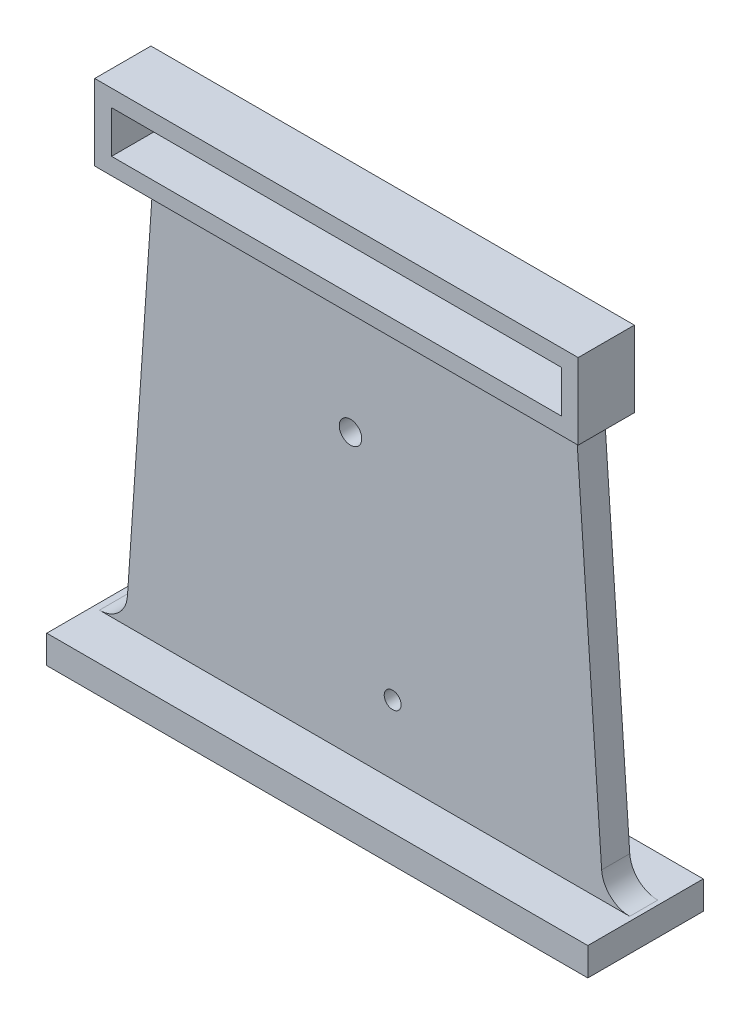
from build123d import *

# Parameters (mm, degrees)
SKETCH1_R           = 3
SKETCH1_R_2         = 4
BOSS_EXTRUDE1_DEPTH = 10
SKETCH2_W           = 192.506357526
SKETCH2_H           = 41.072090777
BOSS_EXTRUDE2_DEPTH = 10
FILLET1_R           = 10
SKETCH3_W           = 172
SKETCH3_H           = 27
SKETCH3_W_2         = 160
SKETCH3_H_2         = 15
BOSS_EXTRUDE3_DEPTH = 10


with BuildPart() as part:
    # Sketch1 → Boss-Extrude1 (new body)
    with BuildSketch(Plane.XY):
        Polygon((0, 0), (170, 0), (160, 146), (10, 146), align=None)
        with Locations((95, 24.5)):
            Circle(SKETCH1_R, mode=Mode.SUBTRACT)
        with Locations((80, 99.5)):
            Circle(SKETCH1_R_2, mode=Mode.SUBTRACT)
    extrude(amount=BOSS_EXTRUDE1_DEPTH)

    # Sketch2 → Boss-Extrude2 (add)
    with BuildSketch(Plane(origin=(0, 0, 0), x_dir=(-1, 0, 0), z_dir=(0, -1, 0))):
        with Locations((-84.638287431, -5.918559418)):
            Rectangle(SKETCH2_W, SKETCH2_H)
    extrude(amount=BOSS_EXTRUDE2_DEPTH)

    # Fillet1
    fillet1_edges = [part.edges().sort_by_distance(p)[0] for p in [
        (170, 0, 5),
        (0, 0, 5),
    ]]
    fillet(fillet1_edges, radius=FILLET1_R)

    # Sketch3 → Boss-Extrude3 (add, symmetric)
    with BuildSketch(Plane.XY.offset(10)):
        with Locations((85, 159.5)):
            Rectangle(SKETCH3_W, SKETCH3_H)
        with Locations((85, 159.5)):
            Rectangle(SKETCH3_W_2, SKETCH3_H_2, mode=Mode.SUBTRACT)
    extrude(amount=BOSS_EXTRUDE3_DEPTH, both=True)


solid = part.part
